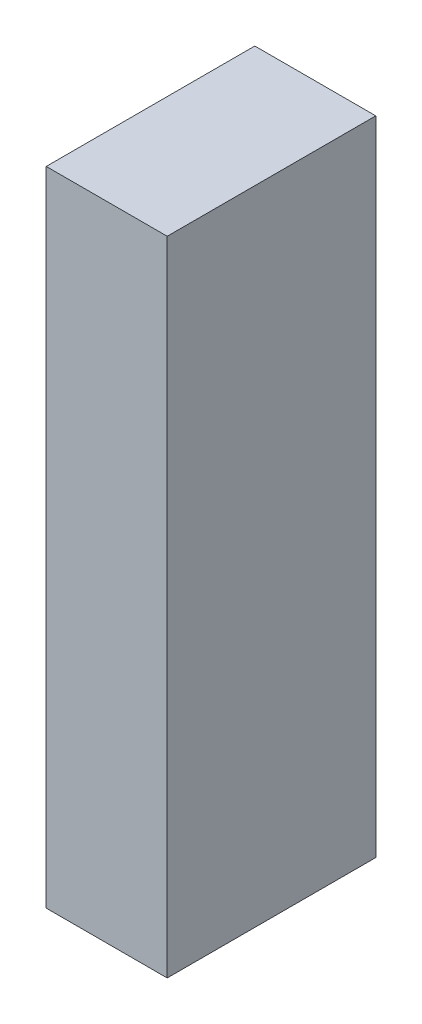
from build123d import *

# Parameters (mm, degrees)
SKETCH1_W           = 14.5
SKETCH1_H           = 77
BOSS_EXTRUDE1_DEPTH = 25


with BuildPart() as part:
    # Sketch1 → Boss-Extrude1 (new body)
    with BuildSketch(Plane.XY):
        Rectangle(SKETCH1_W, SKETCH1_H)
    extrude(amount=BOSS_EXTRUDE1_DEPTH)


solid = part.part
